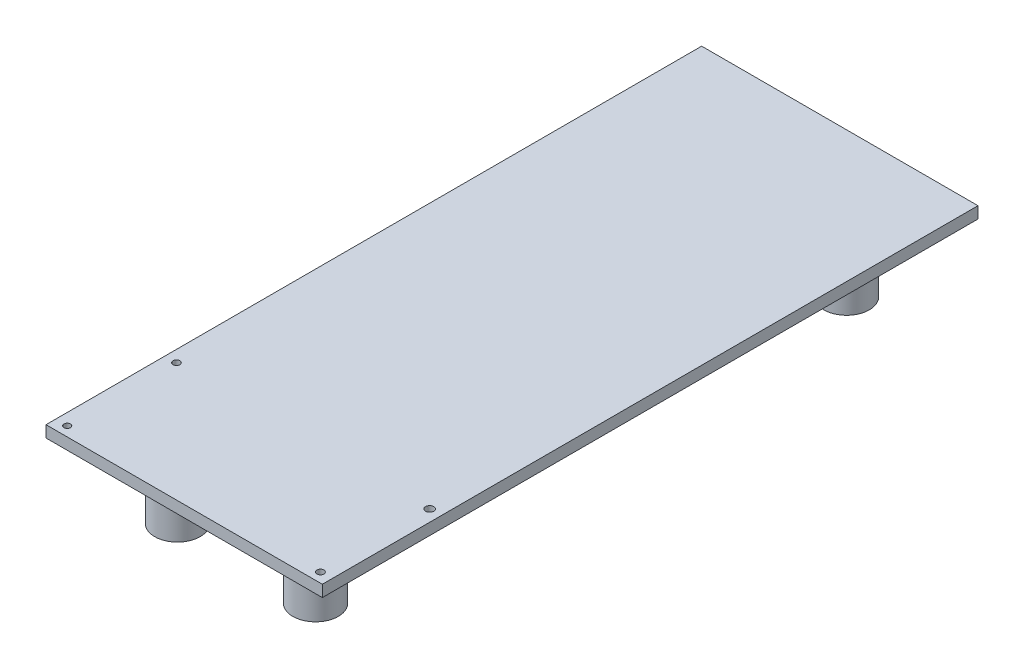
from build123d import *

# Parameters (mm, degrees)
SKETCH1_R           = 5.5
SKETCH1_R_2         = 6.36045924
SKETCH1_R_3         = 5.351214453
SKETCH1_R_4         = 5.079203988
BOSS_EXTRUDE1_DEPTH = 18
SKETCH2_R           = 35.389686151
BOSS_EXTRUDE2_DEPTH = 110


with BuildPart() as part:
    # Sketch1 → Boss-Extrude1 (new body)
    with BuildSketch(Plane(origin=(0, 0, 0), x_dir=(1, 0, 0), z_dir=(0, 1, 0))):
        Polygon((204.197706314, -490.073376619), (-225.802293686, -490.073376619), (-225.802293686, -290.073376619), (-225.802293686, 530.17461365), (204.197706314, 530.17461365), align=None)
        with Locations(Location((186.197706314, -475.073376619, 0), (0, 0, 270))):
            Circle(SKETCH1_R, mode=Mode.SUBTRACT)
        with Locations(Location((186.197706314, -305.073376619, 0), (0, 0, 270))):
            Circle(SKETCH1_R_2, mode=Mode.SUBTRACT)
        with Locations(Location((-207.802293686, -305.073376619, 0), (0, 0, 270))):
            Circle(SKETCH1_R_3, mode=Mode.SUBTRACT)
        with Locations(Location((-207.802293686, -475.073376619, 0), (0, 0, 270))):
            Circle(SKETCH1_R_4, mode=Mode.SUBTRACT)
    extrude(amount=BOSS_EXTRUDE1_DEPTH)

    # Sketch2 → Boss-Extrude2 (add)
    with BuildSketch(Plane.XZ):
        with Locations(Location((96.665522834, 393.073168436, 0), (0, 0, 90))):
            Circle(SKETCH2_R)
        with Locations(Location((-118.270110206, 393.073168436, 0), (0, 0, 90))):
            Circle(SKETCH2_R)
        with Locations(Location((-118.270110206, -433.174405466, 0), (0, 0, 90))):
            Circle(SKETCH2_R)
        with Locations(Location((96.665522834, -433.174405466, 0), (0, 0, 90))):
            Circle(SKETCH2_R)
    extrude(amount=BOSS_EXTRUDE2_DEPTH)


solid = part.part
